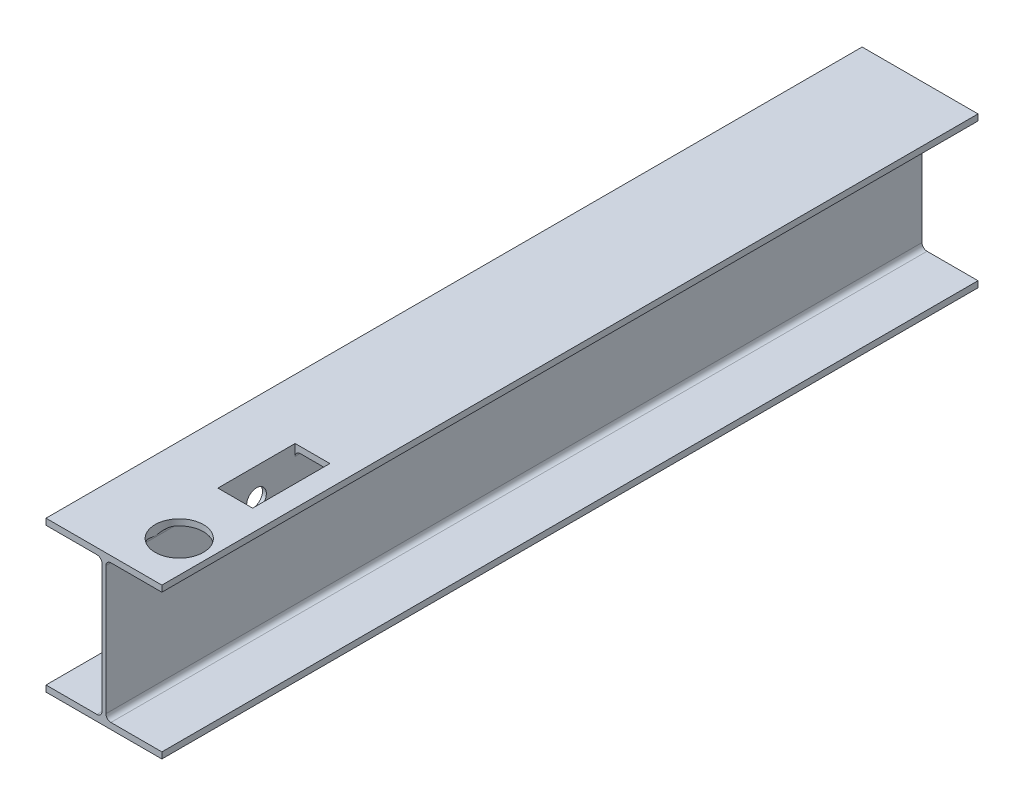
from build123d import *

# Parameters (mm, degrees)
BOSS_EXTRUDE1_DEPTH = 2113
SKETCH2_R           = 62.5
SKETCH2_W           = 90
SKETCH2_H           = 200
CUT_EXTRUDE1_DEPTH  = 30
CUT_EXTRUDE2_REACH  = 2156.273
SKETCH3_R           = 25.5


with BuildPart() as part:
    # Sketch1 → Boss-Extrude1 (new body)
    with BuildSketch(Plane.XY):
        with BuildLine():
            Line((0, 0), (300, 0))
            Line((300, 0), (300, 16))
            Line((300, 16), (168, 16))
            ThreePointArc((168, 16), (158.807611845, 19.807611845), (155, 29))
            Line((155, 29), (155, 361))
            ThreePointArc((155, 361), (158.807611845, 370.192388155), (168, 374))
            Line((168, 374), (300, 374))
            Line((300, 374), (300, 390))
            Line((300, 390), (0, 390))
            Line((0, 390), (0, 374))
            Line((0, 374), (132, 374))
            ThreePointArc((132, 374), (141.192388155, 370.192388155), (145, 361))
            Line((145, 361), (145, 29))
            ThreePointArc((145, 29), (141.192388155, 19.807611845), (132, 16))
            Line((132, 16), (0, 16))
            Line((0, 16), (0, 0))
        make_face()
    extrude(amount=BOSS_EXTRUDE1_DEPTH)

    # Sketch2 → Cut-Extrude1 (cut)
    with BuildSketch(Plane(origin=(0, 390, 0), x_dir=(1, 0, 0), z_dir=(0, 1, 0))):
        with Locations(Location((218, -1986, 0), (0, 0, 270))):
            Circle(SKETCH2_R)
        with Locations((200, -1723)):
            Rectangle(SKETCH2_W, SKETCH2_H)
    extrude(amount=-CUT_EXTRUDE1_DEPTH, mode=Mode.SUBTRACT)

    # Sketch3 → Cut-Extrude2 (cut, up to next)
    with BuildSketch(Plane(origin=(155, 0, 0), x_dir=(0, 0, -1), z_dir=(1, 0, 0)), mode=Mode.PRIVATE) as cut_extrude2_sk1:
        with Locations((-1723, 315)):
            Circle(SKETCH3_R)
    cut_extrude2_tool1 = extrude(cut_extrude2_sk1.sketch, amount=-CUT_EXTRUDE2_REACH, mode=Mode.PRIVATE) & part.part
    add(cut_extrude2_tool1.solids().sort_by_distance((155, 315, 1723))[0], mode=Mode.SUBTRACT)


solid = part.part
